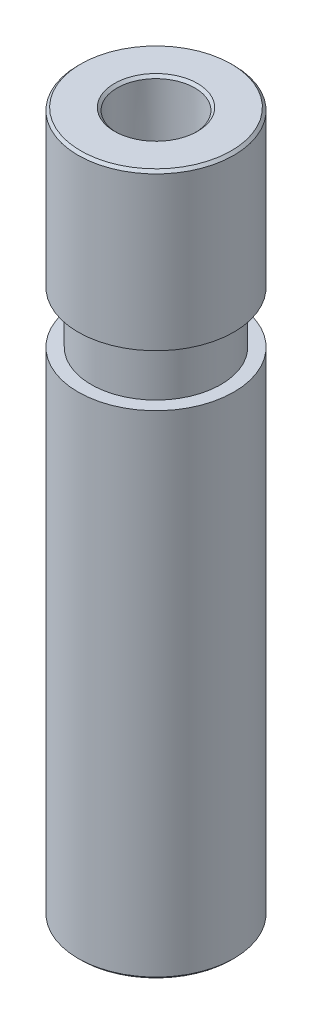
SolidWorks part; units mm, degrees
material "1060 Alloy"
ref_plane "Front Plane" through (0, 0, 0) normal (0, 0, 1) x (1, 0, 0)
ref_plane "Top Plane" through (0, 0, 0) normal (0, 1, 0) x (1, 0, 0)
ref_plane "Right Plane" through (0, 0, 0) normal (1, 0, 0) x (0, 0, -1)
sketch "Sketch1" plane through (0, 0, 0) normal (0, 0, 1) x (1, 0, 0)
  line L0 (0, 0) -> (0, 27) construction
  line L1 (1.1, 0) -> (2.9, 0)
  line L2 (3, 0.1) -> (3, 19)
  line L3 (2.9, 27) -> (1.6, 27)
  line L4 (1.0019, 0.1) -> (1.4981, 26.9)
  line L5 (3, 26.9) -> (2.9, 27)
  line L6 (2.9, 0) -> (3, 0.1)
  line L7 (1.0019, 0.1) -> (1.1, 0)
  line L8 (1.6, 27) -> (1.4981, 26.9)
  line L9 (3, 21) -> (3, 26.9)
  line L10 (3, 21) -> (2.5, 21)
  line L11 (3, 19) -> (2.5, 19)
  line L12 (2.5, 21) -> (2.5, 19)
  point P3 (1, 0)
  point P4 (3, 0)
  point P6 (3, 27)
  point P7 (1.5, 27)
  dimension "D1" = 27
  dimension "D2" = 1
  dimension "D3" = 3
  dimension "D4" = 6
  dimension "D5" = 2
  dimension "D6" = 0.5
  dimension "D7" = 6
revolve "Revolve1" add sketch "Sketch1" angle 360 about L0
